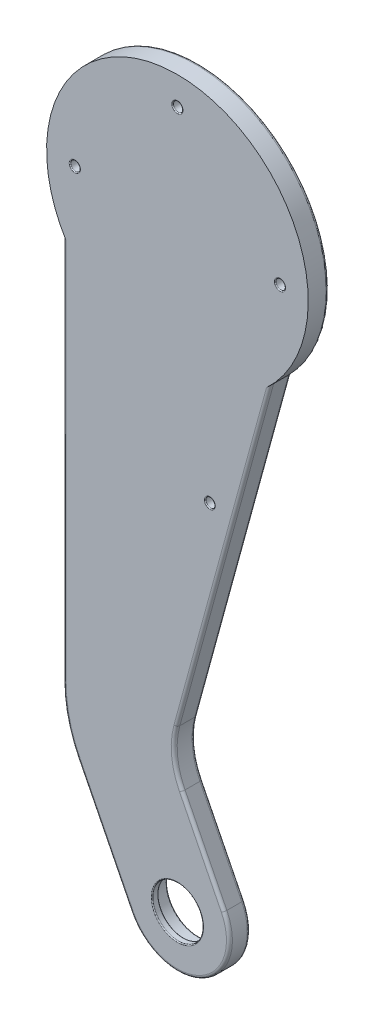
from build123d import *

# Parameters (mm, degrees)
SKETCH1_R           = 8.5
SKETCH1_R_2         = 1.6
BOSS_EXTRUDE1_DEPTH = 7
FILLET1_R           = 25
FILLET2_R           = 45
SKETCH2_R           = 10.5
CUT_EXTRUDE1_DEPTH  = 5
CUT_EXTRUDE2_REACH  = 224.016
SKETCH3_R           = 1.55
SKETCH5_R           = 3.5
CUT_EXTRUDE4_DEPTH  = 1.8
FILLET3_R           = 1
FILLET5_R           = 0.3
FILLET6_R           = 0.1


with BuildPart() as part:
    # Sketch1 → Boss-Extrude1 (new body)
    with BuildSketch(Plane.XY):
        with BuildLine():
            Line((-38.404069543, -21.473878143), (-38.404069543, -162.468720195))
            Line((-38.404069543, -162.468720195), (-15.642417773, -207.846321828))
            ThreePointArc((-15.642417773, -207.846321828), (7.846321828, -215.642417773), (15.642417773, -192.153678172))
            Line((15.642417773, -192.153678172), (-2.725328205, -155.535761851))
            Line((-2.725328205, -155.535761851), (31.378371719, -30.8447368))
            ThreePointArc((31.378371719, -30.8447368), (5.856052892, 43.608561597), (-38.404069543, -21.473878143))
        make_face()
        with Locations((0, -200)):
            Circle(SKETCH1_R, mode=Mode.SUBTRACT)
        with Locations((-34.5, 0)):
            Circle(SKETCH1_R_2, mode=Mode.SUBTRACT)
        with Locations((0, 34.5)):
            Circle(SKETCH1_R_2, mode=Mode.SUBTRACT)
        with Locations((34.5, 0)):
            Circle(SKETCH1_R_2, mode=Mode.SUBTRACT)
    extrude(amount=BOSS_EXTRUDE1_DEPTH)

    # Fillet1
    fillet1_edges = [part.edges().sort_by_distance(p)[0] for p in [
        (-2.725328205, -155.535761851, 3.5),
    ]]
    fillet(fillet1_edges, radius=FILLET1_R)

    # Fillet2
    fillet2_edges = [part.edges().sort_by_distance(p)[0] for p in [
        (-38.404069543, -162.468720195, 3.5),
    ]]
    fillet(fillet2_edges, radius=FILLET2_R)

    # Sketch2 → Cut-Extrude1 (cut)
    with BuildSketch(Plane(origin=(0, 0, 0), x_dir=(-1, 0, 0), z_dir=(0, 0, -1))):
        with Locations((0, -200)):
            Circle(SKETCH2_R)
    extrude(amount=-CUT_EXTRUDE1_DEPTH, mode=Mode.SUBTRACT)

    # Sketch3 → Cut-Extrude2 (cut, up to next)
    with BuildSketch(Plane.XY.offset(7), mode=Mode.PRIVATE) as cut_extrude2_sk1:
        with Locations((10.909211738, -75.36057928)):
            Circle(SKETCH3_R)
    cut_extrude2_tool1 = extrude(cut_extrude2_sk1.sketch, amount=-CUT_EXTRUDE2_REACH, mode=Mode.PRIVATE) & part.part
    add(cut_extrude2_tool1.solids().sort_by_distance((10.909212, -75.360579, 7))[0], mode=Mode.SUBTRACT)

    # Sketch5 → Cut-Extrude4 (cut)
    with BuildSketch(Plane(origin=(0, 0, 0), x_dir=(-1, 0, 0), z_dir=(0, 0, -1))):
        with Locations((0, 34.5)):
            Circle(SKETCH5_R)
        with Locations((-10.909211738, -75.36057928)):
            Circle(SKETCH5_R)
        with Locations((34.5, 0)):
            Circle(SKETCH5_R)
        with Locations((-34.5, 0)):
            Circle(SKETCH5_R)
    extrude(amount=-CUT_EXTRUDE4_DEPTH, mode=Mode.SUBTRACT)

    # Fillet3
    fillet3_edges = [part.edges().sort_by_distance(p)[0] for p in [
        (7.846321828, -215.642417773, 0),
        (-38.404069543, -86.644523001, 0),
        (5.856052892, 43.608561597, 0),
        (15.590252243, -88.569757998, 0),
        (15.590252243, -88.569757998, 7),
        (8.606281967, -178.12644628, 0),
        (8.606281967, -178.12644628, 7),
        (-0.961186177, -155.36057928, 0),
        (-0.961186177, -155.36057928, 7),
        (-38.404069543, -86.644523001, 7),
        (-24.634923651, -189.918872908, 0),
        (-24.634923651, -189.918872908, 7),
        (-37.19362994, -162.182153935, 0),
        (-37.19362994, -162.182153935, 7),
        (7.846321828, -215.642417773, 7),
    ]]
    fillet(fillet3_edges, radius=FILLET3_R)

    # Fillet5
    fillet5_edges = [part.edges().sort_by_distance(p)[0] for p in [
        (32.9, 0, 7),
        (-36.1, 0, 7),
        (-8.5, -200, 7),
        (-1.6, 34.5, 7),
        (10.5, -200, 0),
        (9.359211738, -75.36057928, 7),
        (3.5, 34.5, 0),
        (14.409211738, -75.36057928, 0),
        (-31, 0, 0),
        (38, 0, 0),
    ]]
    fillet(fillet5_edges, radius=FILLET5_R)

    # Fillet6
    fillet6_edges = [part.edges().sort_by_distance(p)[0] for p in [
        (10.5, -200, 5),
        (-8.5, -200, 5),
        (3.5, 34.5, 1.8),
        (-1.6, 34.5, 1.8),
        (14.409211738, -75.36057928, 1.8),
        (9.359211738, -75.36057928, 1.8),
        (-31, 0, 1.8),
        (-36.1, 0, 1.8),
        (38, 0, 1.8),
        (32.9, 0, 1.8),
    ]]
    fillet(fillet6_edges, radius=FILLET6_R)


solid = part.part
